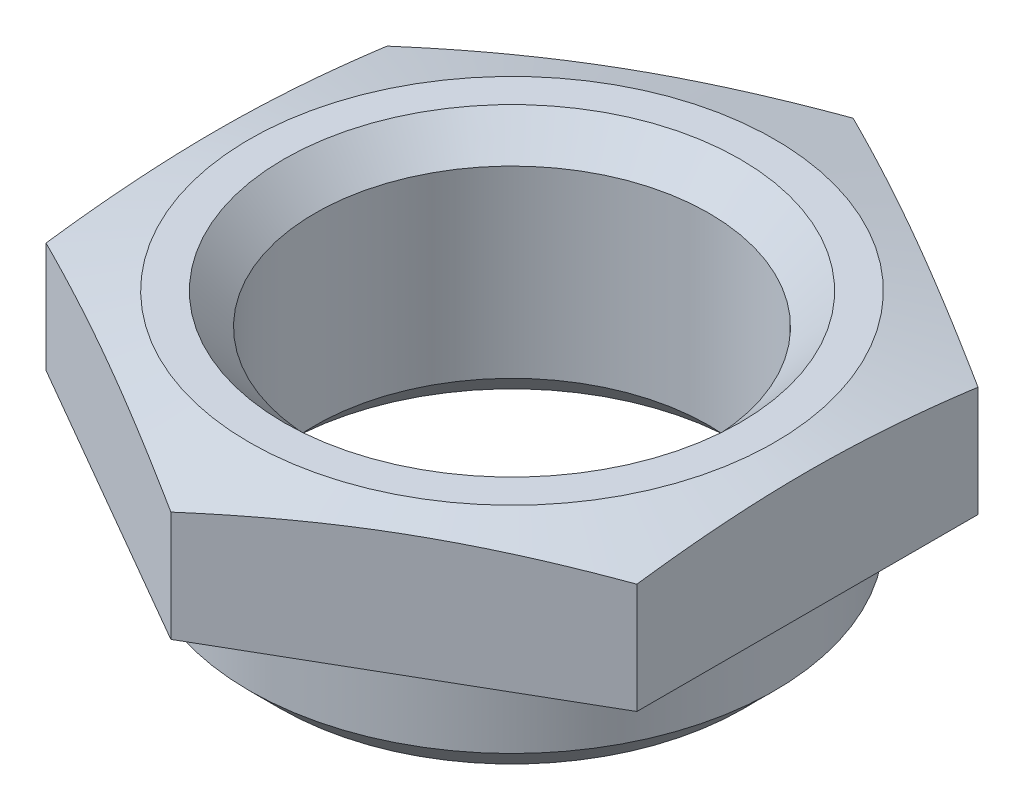
SolidWorks part; units mm, degrees
ref_plane "前视基准面" through (0, 0, 0) normal (0, 0, 1) x (1, 0, 0)
ref_plane "上视基准面" through (0, 0, 0) normal (0, 1, 0) x (1, 0, 0)
ref_plane "右视基准面" through (0, 0, 0) normal (1, 0, 0) x (0, 0, -1)
sketch "草图1" plane through (0, 0, 0) normal (0, 0, 1) x (1, 0, 0)
  line L0 (0, 0) -> (0, -6.0355) construction
  line L1 (-13.9, 0) -> (-14.1, 0)
  line L2 (-14.1, 0) -> (-16, 1.9)
  line L3 (-16, 1.9) -> (-16, 7)
  line L4 (-16, 7) -> (-18, 7)
  line L5 (-18, 7) -> (-18, 14.4641)
  line L6 (-18, 14.4641) -> (-16, 15)
  line L7 (-16, 15) -> (-13.9, 15)
  line L8 (-13.9, 15) -> (-12, 13.1)
  line L9 (-12, 13.1) -> (-12, 1.9)
  line L10 (-12, 1.9) -> (-13.9, 0)
  point P3 (-12, 0)
revolve "旋转1" add sketch "草图1" angle 360 about L0
sketch "草图2" plane through (0, 15, 0) normal (0, 1, 0) x (1, 0, 0)
  line L1 (18, -10.3923) -> (18, 10.3923)
  line L2 (18, 10.3923) -> (0, 20.7846)
  line L3 (0, 20.7846) -> (-18, 10.3923)
  line L4 (-18, 10.3923) -> (-18, -10.3923)
  line L5 (-18, -10.3923) -> (0, -20.7846)
  line L6 (0, -20.7846) -> (18, -10.3923)
  circle A0 centre (0, 0) radius 18 construction
  circle A1 centre (0, 0) radius 18 construction
extrude "拉伸1" add sketch "草图2" against normal up to vertex (8 mm away) up to point (-18, 7, 0)
sketch "草图3" plane through (0, 0, 0) normal (0, 0, 1) x (1, 0, 0)
  line L0 (-29.9, 11.2755) -> (-16, 15)
  line L1 (-16, 15) -> (-29.9, 15)
  line L4 (-29.9, 15) -> (-29.9, 11.2755)
  line L5 (0, 0) -> (0, -7.8437) construction
  line L7 (-18, 14.4641) -> (-16, 15) construction
  line L8 (-13.9, 15) -> (-12, 13.1)
  line L9 (-12, 13.1) -> (-12, 0)
  line L10 (-12, 0) -> (0, 0)
  line L11 (0, 0) -> (0, 15)
  line L12 (0, 15) -> (-13.9, 15)
revolve "切除-旋转2" cut sketch "草图3" angle 360 about L5
equation "\"D11@草图1\" =\"cm@草图1\""
